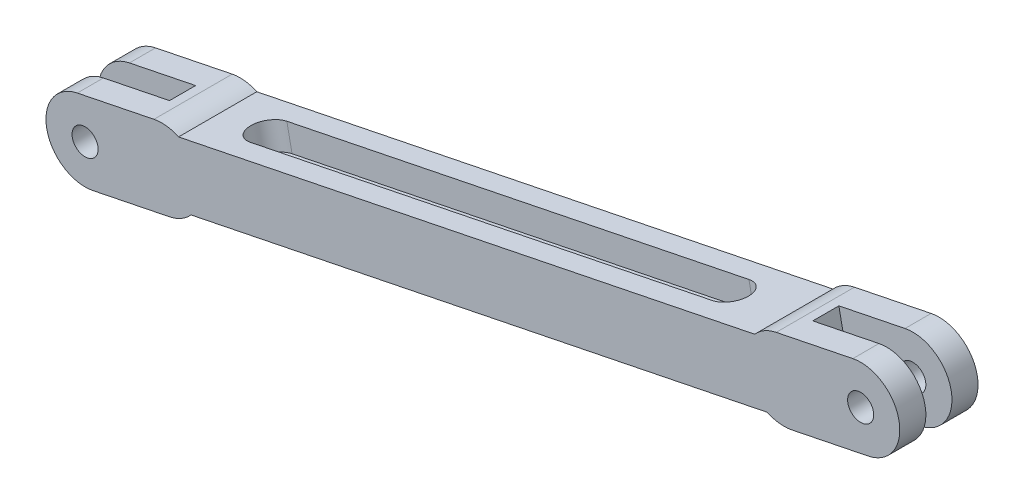
from build123d import *

# Parameters (mm, degrees)
BOSS_EXTRUDE1_DEPTH = 30
SKETCH2_W           = 45.814700403
SKETCH2_H           = 10
CUT_EXTRUDE1_DEPTH  = 80
CUT_EXTRUDE2_DEPTH  = 10


with BuildPart() as part:
    # Sketch1 → Boss-Extrude1 (new body)
    with BuildSketch(Plane.XY.offset(3001.335718486)):
        with BuildLine():
            Line((917.934929034, 337.734430273), (888.537204265, 331.753311783))
            ThreePointArc((888.537204265, 331.753311783), (884.042481487, 330.053316774), (880.315998683, 327.019203759))
            Line((880.315998683, 327.019203759), (659.406795905, 282.074088861))
            ThreePointArc((659.406795905, 282.074088861), (654.791020678, 283.41092652), (649.989366626, 283.21952579))
            Line((649.989366626, 283.21952579), (620.591641856, 277.2384073))
            ThreePointArc((620.591641856, 277.2384073), (608.883338717, 259.54898567), (626.572760347, 247.840682531))
            Line((626.572760347, 247.840682531), (655.970485116, 253.821801021))
            ThreePointArc((655.970485116, 253.821801021), (660.465207894, 255.521796031), (664.191690698, 258.555909045))
            Line((664.191690698, 258.555909045), (885.100893475, 303.501023943))
            ThreePointArc((885.100893475, 303.501023943), (889.716668703, 302.164186284), (894.518322755, 302.355587014))
            Line((894.518322755, 302.355587014), (923.916047524, 308.336705504))
            ThreePointArc((923.916047524, 308.336705504), (935.624350664, 326.026127134), (917.934929034, 337.734430273))
        make_face()
        with BuildLine():
            ThreePointArc((618.682580307, 261.542691833), (624.579054184, 257.63992412), (628.481821897, 263.536397997))
            ThreePointArc((628.481821897, 263.536397997), (622.58534802, 267.43916571), (618.682580307, 261.542691833))
        make_face(mode=Mode.SUBTRACT)
        with BuildLine():
            ThreePointArc((916.025867484, 322.038714807), (921.922341361, 318.135947094), (925.825109074, 324.032420971))
            ThreePointArc((925.825109074, 324.032420971), (919.928635197, 327.935188684), (916.025867484, 322.038714807))
        make_face(mode=Mode.SUBTRACT)
    extrude(amount=-BOSS_EXTRUDE1_DEPTH)

    # Sketch2 → Cut-Extrude1 (cut)
    with BuildSketch(Plane(origin=(-23.514742418, 115.577032406, 0), x_dir=(0.9799241589705207, 0.19937061635536468, 0), z_dir=(0.19937061635536468, -0.9799241589705207, 0))):
        with Locations((963.863089214, 2986.335718486)):
            Rectangle(SKETCH2_W, SKETCH2_H)
        with Locations((666.383780489, 2986.335718486)):
            Rectangle(SKETCH2_W, SKETCH2_H)
    extrude(amount=-CUT_EXTRUDE1_DEPTH, mode=Mode.SUBTRACT)

    # Sketch3 → Cut-Extrude2 (cut)
    with BuildSketch(Plane(origin=(-24.112854267, 118.516804882, 0), x_dir=(0.9799241589705208, 0.19937061635536377, 0), z_dir=(0.19937061635536377, -0.9799241589705208, 0))):
        with BuildLine():
            Line((722.337924675, 2993.335718486), (903.120015469, 2993.335718486))
            ThreePointArc((903.120015469, 2993.335718486), (910.120015469, 2986.335718486), (903.120015469, 2979.335718486))
            Line((903.120015469, 2979.335718486), (722.337924675, 2979.335718486))
            ThreePointArc((722.337924675, 2979.335718486), (715.337924675, 2986.335718486), (722.337924675, 2993.335718486))
        make_face()
    cut_extrude2 = extrude(amount=-CUT_EXTRUDE2_DEPTH, mode=Mode.SUBTRACT)

    # Mirror1: Cut-Extrude2 across plane
    add(cut_extrude2.mirror(Plane(origin=(-26.505301663, 130.27589479, 0), x_dir=(0, 0, 1), z_dir=(0.1993706163553639, -0.9799241589705208, 0))), mode=Mode.SUBTRACT)


solid = part.part
